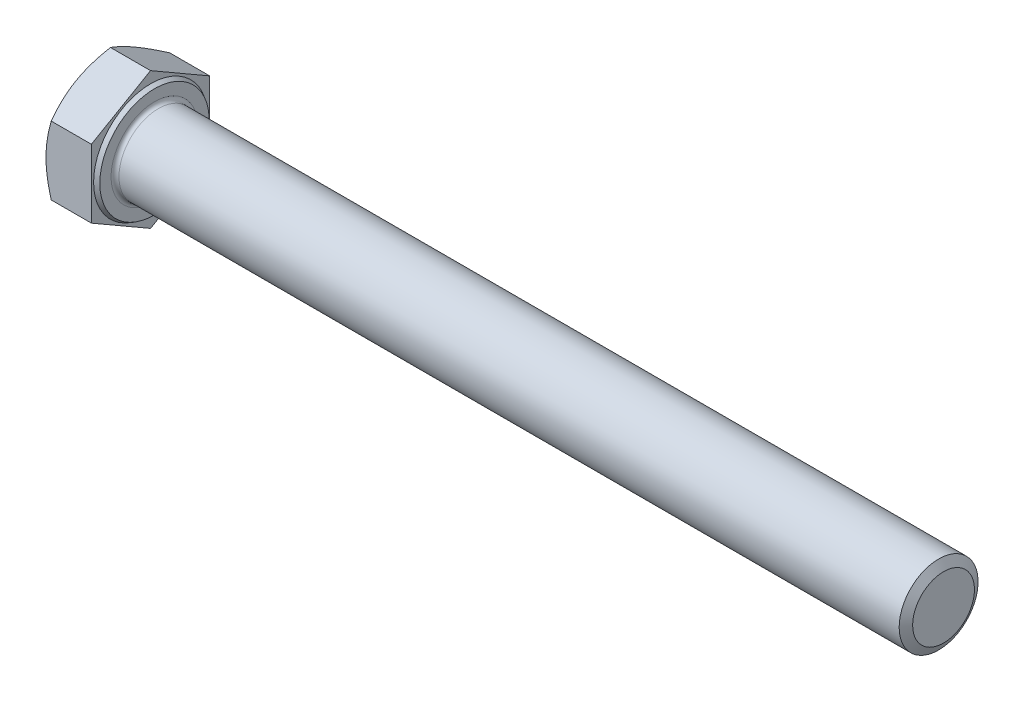
SolidWorks part; units mm, degrees
ref_plane "前视" through (0, 0, 0) normal (0, 0, 1) x (1, 0, 0)
ref_plane "上视" through (0, 0, 0) normal (0, 1, 0) x (1, 0, 0)
ref_plane "右视" through (0, 0, 0) normal (1, 0, 0) x (0, 0, -1)
sketch "草图1" plane through (0, 0, 0) normal (1, 0, 0) x (0, 0, -1)
  line L0 (9, 5.1962) -> (9, -5.1962)
  line L1 (-9, 5.1962) -> (-9, -5.1962)
  line L2 (9, -5.1962) -> (0, -10.3923)
  line L3 (0, -10.3923) -> (-9, -5.1962)
  line L4 (9, 5.1962) -> (0, 10.3923)
  line L5 (0, 10.3923) -> (-9, 5.1962)
  circle A0 centre (0, 0) radius 10.015 construction
  dimension "e" = 20.03
  dimension "s" = 18
  dimension "D2" = 120
  dimension "D3" = 9
  dimension "D4" = 9
  dimension "D5" = 9
extrude "基体-拉伸" add sketch "草图1" along normal blind 7.5
sketch "草图2" plane through (0, 0, 0) normal (0, 0, 1) x (1, 0, 0)
  line L0 (0, 5.1962) -> (0, -5.1962) construction
  line L1 (0, 0) -> (127.5, 0)
  line L2 (0, 0) -> (0, 6)
  line L3 (0, 6) -> (63.75, 6)
  line L4 (127.5, 0) -> (127.5, 4.701)
  line L5 (7.5, 10.3923) -> (7.5, 5.1962) construction
  line L6 (0, 0) -> (-13.7, 0) construction
  line L7 (0, 0) -> (96.52, 0) construction
  line L8 (127.5, -4.701) -> (63.75, -6) construction
  line L9 (0, -6) -> (63.75, -6) construction
  line L10 (9, 15.24) -> (9, -1.27) construction
  line L11 (7.5, 15.24) -> (7.5, -1.27) construction
  line L12 (7.5, 5.1962) -> (7.5, -5.1962) construction
  line L13 (63.75, 6) -> (127.5, 6)
  line L14 (127.5, 6) -> (127.5, 4.701)
  line L15 (-13.7, 0) -> (-13.7, 20) construction
  dimension "l" = 120
  dimension "d" = 12
  dimension "Minor_dia" = 9.402
  dimension "p" = 1.5
  dimension "b" = 120
  dimension "da" = 13.7
  dimension "ds" = 20
revolve "凸台-旋转1" add sketch "草图2" angle 360 about L7
cosmetic thread "螺旋线1" parameters "Thread_length"=120, "Thread_minor"=9.402
sketch "草图3" plane through (0, 0, 0) normal (0, 0, 1) x (1, 0, 0)
  line L0 (0, 9) -> (3.6906, 15.3923)
  line L1 (0, 10.3923) -> (0, 5.1962) construction
  line L2 (3.6906, 15.3923) -> (3.6906, 20.3923)
  line L3 (3.6906, 20.3923) -> (-10, 20.3923)
  line L4 (-10, 20.3923) -> (-10, 9)
  line L5 (-10, 9) -> (0, 9)
  line L6 (0, 0) -> (99.06, 0) construction
  line L7 (7.5, 10.3923) -> (0, 10.3923) construction
  dimension "D1" = 9
  dimension "D2" = 5
  dimension "D3" = 10
  dimension "D4" = 5
  dimension "Head_ch_ang" = 30
revolve "切除-旋转1" cut sketch "草图3" angle 360 about L6
sketch "草图4" plane through (0, 0, 0) normal (0, 0, 1) x (1, 0, 0)
  line L0 (0, 0) -> (216.8159, 0) construction
  line L2 (7.5, 0) -> (7.5, 8.315) construction
  line L9 (7.5, -6) -> (7.5, 6) construction
  line L10 (7.5, 10.3923) -> (7.5, 5.1962) construction
  line L11 (7.5, 8.315) -> (6.9, 8.6614)
  line L12 (6.9, 8.6614) -> (6.9, 10.3923)
  line L13 (7.5, 10.3923) -> (0.8038, 10.3923) construction
  line L14 (6.9, 10.3923) -> (7.5, 10.3923)
  line L15 (7.5, 10.3923) -> (7.5, 8.315)
  dimension "D1" = 120
  dimension "c" = 0.6
  dimension "dw" = 16.63
revolve "切除-旋转3" cut sketch "草图4" angle 360 about L0
fillet "圆角" radius 0.6 1 edges at (7.5, 0, -6)
sketch "草图6" plane through (0, 0, 0) normal (0, 0, 1) x (1, 0, 0)
  line L0 (0, 0) -> (127.5, 0) construction
  line L1 (127.5, -6) -> (127.5, 6) construction
  line L2 (127.5, 0) -> (127.5, 6) construction
  line L4 (126.75, 6) -> (128.25, 6)
  line L5 (126.75, 6) -> (127.5, 4.701)
  line L6 (127.5, 4.701) -> (128.25, 6)
  dimension "D1" = 1.5
revolve "切除-旋转4" cut sketch "草图6" angle 360 about L0
pattern_linear "阵列(线性)1" [suppressed]
